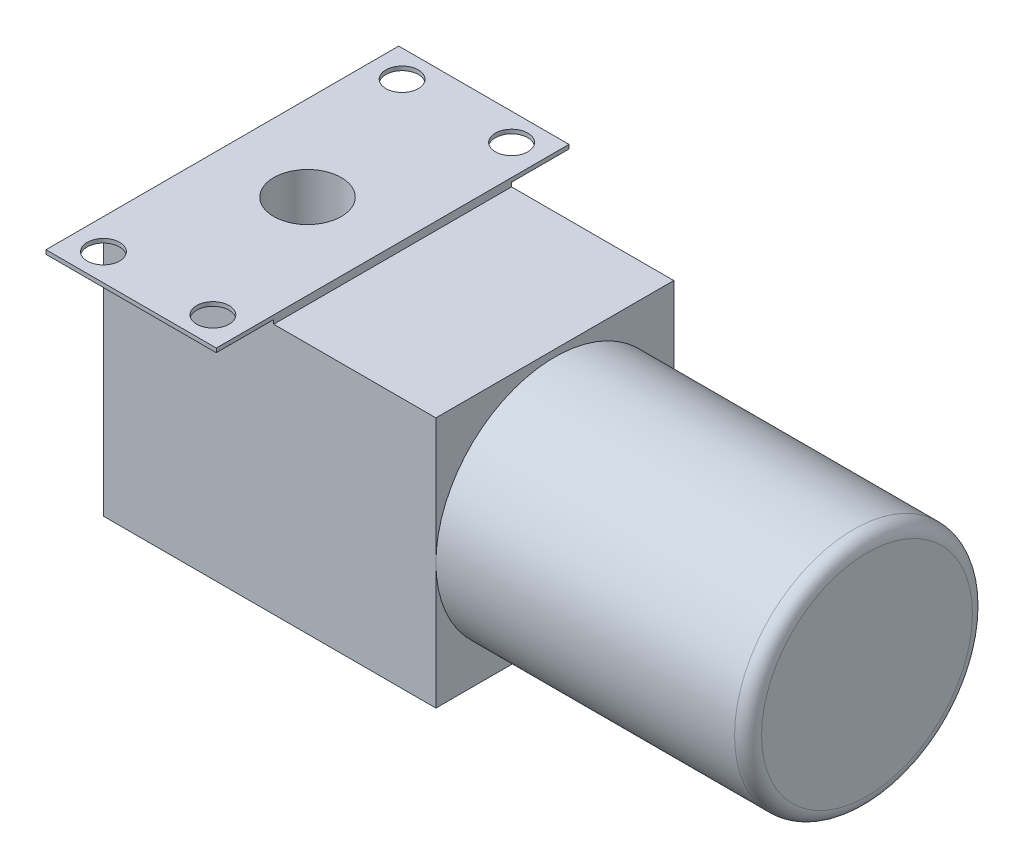
from build123d import *

# Parameters (mm, degrees)
SKETCH_1_W          = 63
SKETCH_1_H          = 130.5
EXTRUDE_1_DEPTH     = 1.5
EXTRUDE_START       = 1.5
SKETCH_2_W          = 123
SKETCH_2_H          = 88
EXTRUDE_2_DEPTH     = 93
SKETCH_3_R          = 44
EXTRUDE_3_DEPTH     = 115.5
SKETCH_5_W          = 63
SKETCH_5_H          = 88
EXTRUDE_4_DEPTH     = 3
SKETCH_6_R          = 6
CUT_EXTRUDE_2_DEPTH = 238.323750392
SKETCH_4_R          = 12.5
CUT_EXTRUDE_1_DEPTH = 238.323750392
FILLET_1_R          = 5


with BuildPart() as part:
    # 草图1 → 凸台-拉伸1 (new body)
    with BuildSketch(Plane(origin=(0, 0, 0), x_dir=(1, 0, 0), z_dir=(0, 1, 0))):
        Rectangle(SKETCH_1_W, SKETCH_1_H)
    extrude(amount=EXTRUDE_1_DEPTH)



with BuildPart() as body_2:
    # 草图2 → 凸台-拉伸2 (new body)
    with BuildSketch(Plane.XZ.offset(EXTRUDE_START)):
        with Locations((30, 0)):
            Rectangle(SKETCH_2_W, SKETCH_2_H)
    extrude(amount=EXTRUDE_2_DEPTH)

    # 草图3 → 凸台-拉伸3 (add)
    with BuildSketch(Plane(origin=(91.5, 0, 0), x_dir=(0, 0, -1), z_dir=(1, 0, 0))):
        with Locations((0, -48)):
            Circle(SKETCH_3_R)
    extrude(amount=EXTRUDE_3_DEPTH)


with BuildPart() as part_1:
    add(part.part)

    add(body_2.part)  # 凸台-拉伸4 merges body 2
    # 草图5 → 凸台-拉伸4 (add)
    with BuildSketch(Plane.XZ):
        Rectangle(SKETCH_5_W, SKETCH_5_H)
    extrude(amount=EXTRUDE_4_DEPTH)

    # 草图6 → 切除-拉伸2 (cut, through all)
    with BuildSketch(Plane(origin=(0, 1.5, 0), x_dir=(1, 0, 0), z_dir=(0, 1, 0))):
        with Locations(Location((-20.25, 55.25, 0), (0, 0, 270))):
            Circle(SKETCH_6_R)
        with Locations(Location((20.25, 55.25, 0), (0, 0, 270))):
            Circle(SKETCH_6_R)
        with Locations(Location((-20.25, -55.25, 0), (0, 0, 270))):
            Circle(SKETCH_6_R)
        with Locations(Location((20.25, -55.25, 0), (0, 0, 270))):
            Circle(SKETCH_6_R)
    extrude(amount=-CUT_EXTRUDE_2_DEPTH, mode=Mode.SUBTRACT)

    # 草图4 → 切除-拉伸1 (cut, through all)
    with BuildSketch(Plane(origin=(0, 1.5, 0), x_dir=(1, 0, 0), z_dir=(0, 1, 0))):
        with Locations(Location((0, 0, 0), (0, 0, 270))):
            Circle(SKETCH_4_R)
    extrude(amount=-CUT_EXTRUDE_1_DEPTH, mode=Mode.SUBTRACT)

    # 圆角1
    fillet_1_edges = [part_1.edges().sort_by_distance(p)[0] for p in [
        (207, -48, 44),
    ]]
    fillet(fillet_1_edges, radius=FILLET_1_R)


solid = part_1.part
